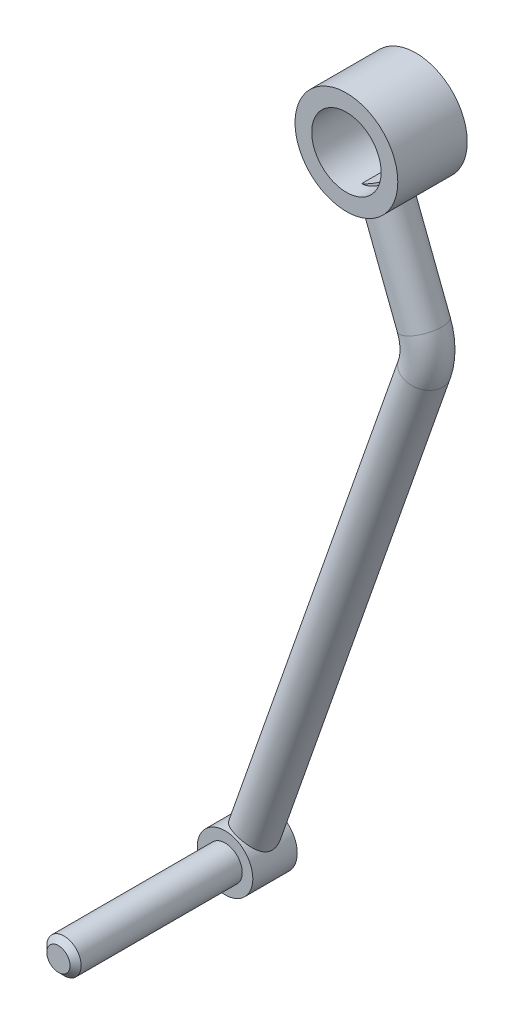
SolidWorks part; units mm, degrees
material "AISI 304"
ref_plane "Front Plane" through (0, 0, 0) normal (0, 0, 1) x (1, 0, 0)
ref_plane "Top Plane" through (0, 0, 0) normal (0, 1, 0) x (1, 0, 0)
ref_plane "Right Plane" through (0, 0, 0) normal (1, 0, 0) x (0, 0, -1)
sketch "Sketch1" plane through (0, 0, 0) normal (0, 0, 1) x (1, 0, 0)
  circle A0 centre (0, 0) radius 6.25
  circle A1 centre (0, 0) radius 9.25
  dimension "D1" = 12.5
  dimension "D2" = 3
extrude "Boss-Extrude1" add sketch "Sketch1" along normal blind 12.5
sketch3d "3DSketch1"
  line L0 (0, -6.25, 6.25) -> (7.6754, -26.1378, 6.25)
  line L1 (7.7824, -33.0482, 6.25) -> (-24.0974, -123.9368, 6.25)
  line L2 (0, 0, 0) -> (0, -6.25, 0) construction
  line L3 (0, -6.25, 0) -> (0, -6.25, 6.25) construction
  arc A0 (7.7824, -33.0482, 6.25) -> (7.6754, -26.1378, 6.25) centre (-1.6539, -29.7383, 6.25) ccw
  circle A1 centre (0, 0, 0) radius 6.25 construction
  point P5 (9.0013, -29.5733, 6.25)
  point P6 (-1.6539, -29.7383, 16.25)
  point P15 (0, 0, 6.25)
  dimension "D1" = 10
  dimension "D2" = 100
  dimension "D3" = 25
  dimension "D4" = 6.25
sweep "Sweep1" add path "3DSketch1" circular profile diameter 7 parameters "D3"=7
ref_plane "Plane1" through (0, 0, 6.25) normal (0, 0, 1) x (1, 0, 0)
sketch "Sketch16" plane through (0, 0, 6.25) normal (0, 0, 1) x (1, 0, 0)
  line L1 (-27.4002, -122.7784) -> (-20.7947, -125.0953) construction
  circle A1 centre (-24.0974, -123.9368) radius 5
  dimension "D1" = 10
extrude "Boss-Extrude2" add sketch "Sketch16" along normal mid plane 8
sketch "Sketch17" plane through (0, 0, 10.25) normal (0, 0, 1) x (1, 0, 0)
  circle A0 centre (-24.0974, -123.9368) radius 3.0961
extrude "Boss-Extrude3" add sketch "Sketch17" along normal blind 30
chamfer "Chamfer1" distance 1 angle 45 1 edges at (-21.0013, -123.9368, 40.25)
